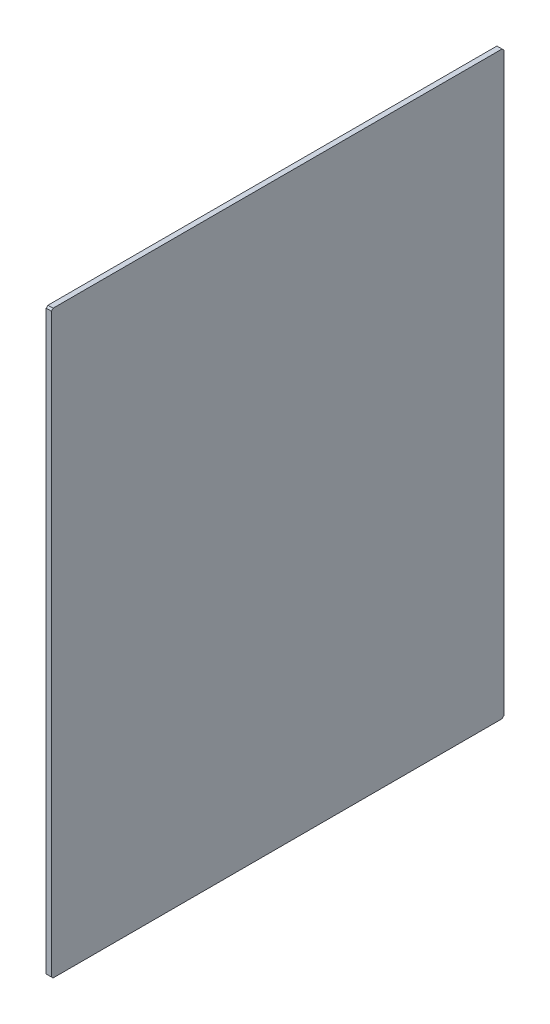
SolidWorks part; units mm, degrees
material "茶色亚克力"
ref_plane "前视基准面" through (0, 0, 0) normal (0, 0, 1) x (1, 0, 0)
ref_plane "上视基准面" through (0, 0, 0) normal (0, 1, 0) x (1, 0, 0)
ref_plane "右视基准面" through (0, 0, 0) normal (1, 0, 0) x (0, 0, -1)
sketch "草图1" plane through (0, 0, 0) normal (1, 0, 0) x (0, 0, -1)
  line L1 (-264, 338.5) -> (264, 338.5)
  line L2 (-264, 338.5) -> (-264, -338.5)
  line L3 (-264, -338.5) -> (264, -338.5)
  line L4 (264, 338.5) -> (264, -338.5)
  line L5 (-264, 338.5) -> (264, -338.5) construction
  line L6 (-264, -338.5) -> (264, 338.5) construction
  point P0 (0, 0)
  dimension "D1" = 528
  dimension "D2" = 677
extrude "凸台-拉伸1" add sketch "草图1" along normal mid plane 6
chamfer "倒角1" distance 2 angle 45 4 edges at (0, -338.5, 264) (0, -338.5, -264) (0, 338.5, -264) (0, 338.5, 264)
